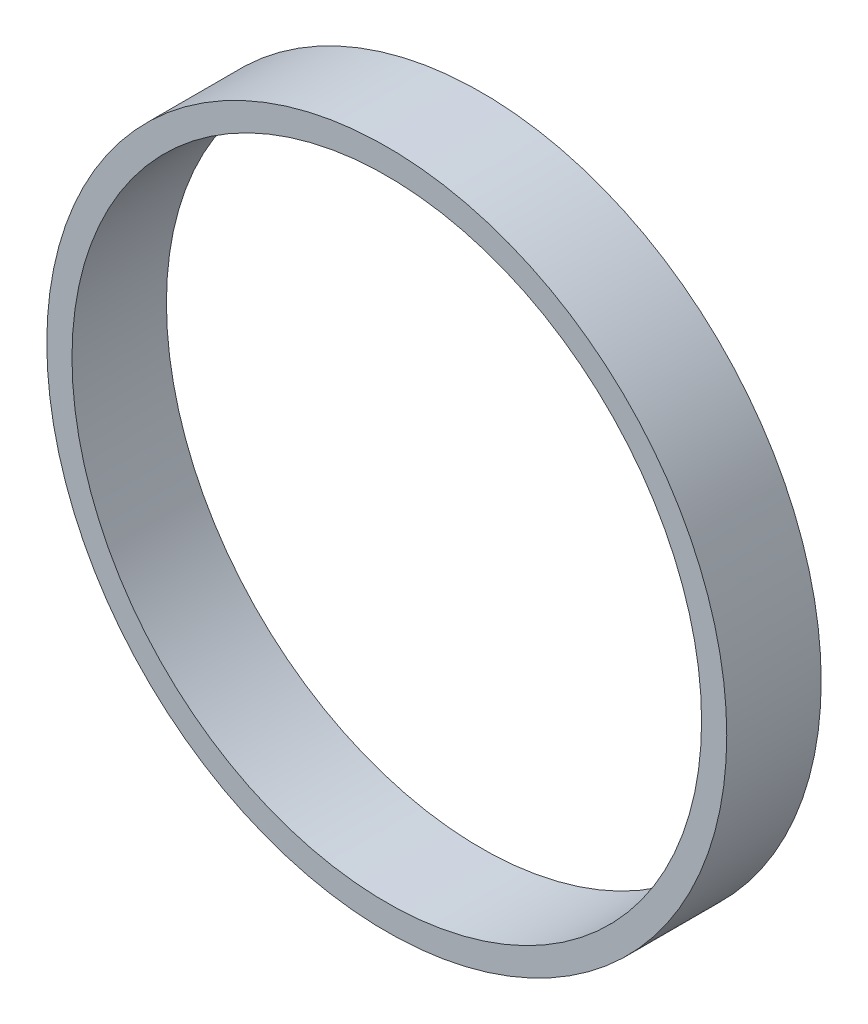
SolidWorks part; units mm, degrees
ref_plane "Front Plane" through (0, 0, 0) normal (0, 0, 1) x (1, 0, 0)
ref_plane "Top Plane" through (0, 0, 0) normal (0, 1, 0) x (1, 0, 0)
ref_plane "Right Plane" through (0, 0, 0) normal (1, 0, 0) x (0, 0, -1)
sketch "Sketch1" plane through (0, 0, 0) normal (0, 0, 1) x (1, 0, 0)
  circle A0 centre (0, 0) radius 54
  circle A2 centre (0, 0) radius 50
  dimension "D1" = 108
  dimension "D2" = 100
extrude "Boss-Extrude1" add sketch "Sketch1" along normal blind 15
